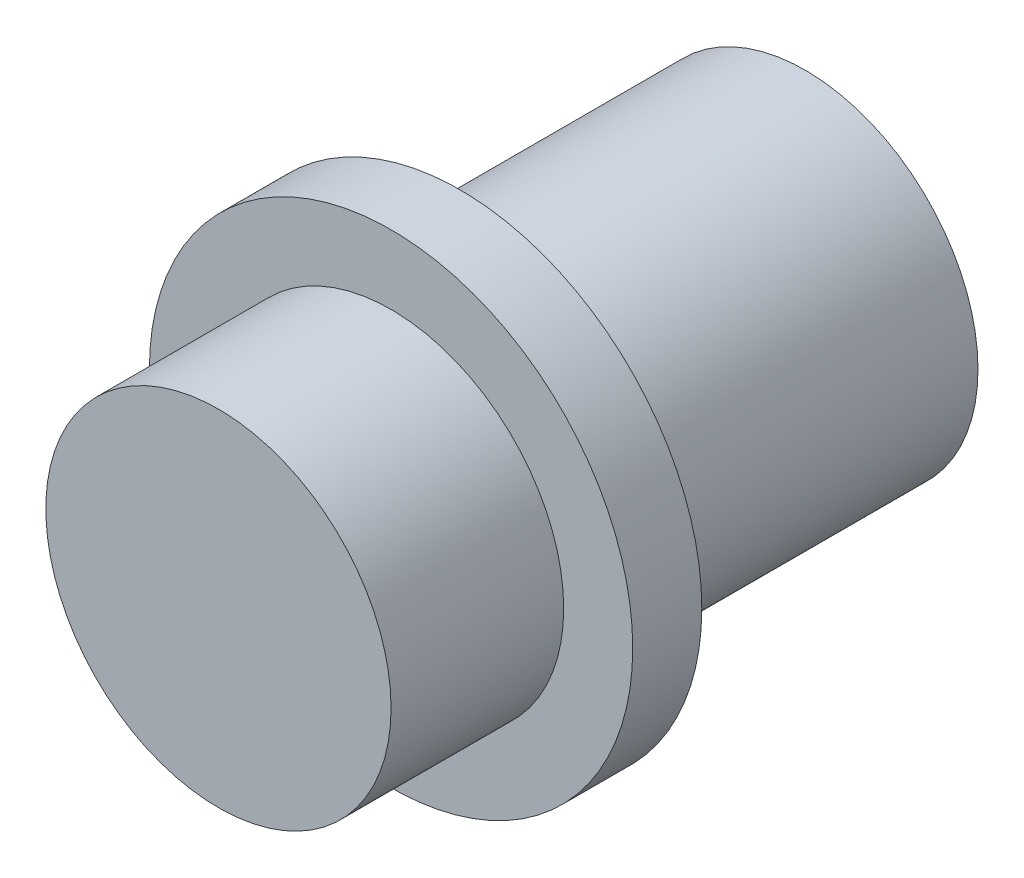
from build123d import *

# Parameters (mm, degrees)
SKETCH1_R           = 5
BOSS_EXTRUDE1_DEPTH = 10
SKETCH2_R           = 7
BOSS_EXTRUDE2_DEPTH = 2
SKETCH4_R           = 5
BOSS_EXTRUDE3_DEPTH = 5


with BuildPart() as part:
    # Sketch1 → Boss-Extrude1 (new body)
    with BuildSketch(Plane.XY):
        Circle(SKETCH1_R)
    extrude(amount=BOSS_EXTRUDE1_DEPTH)

    # Sketch2 → Boss-Extrude2 (add)
    with BuildSketch(Plane.XY.offset(10)):
        Circle(SKETCH2_R)
    extrude(amount=BOSS_EXTRUDE2_DEPTH)

    # Sketch4 → Boss-Extrude3 (add)
    with BuildSketch(Plane.XY.offset(12)):
        Circle(SKETCH4_R)
    extrude(amount=BOSS_EXTRUDE3_DEPTH)


solid = part.part
